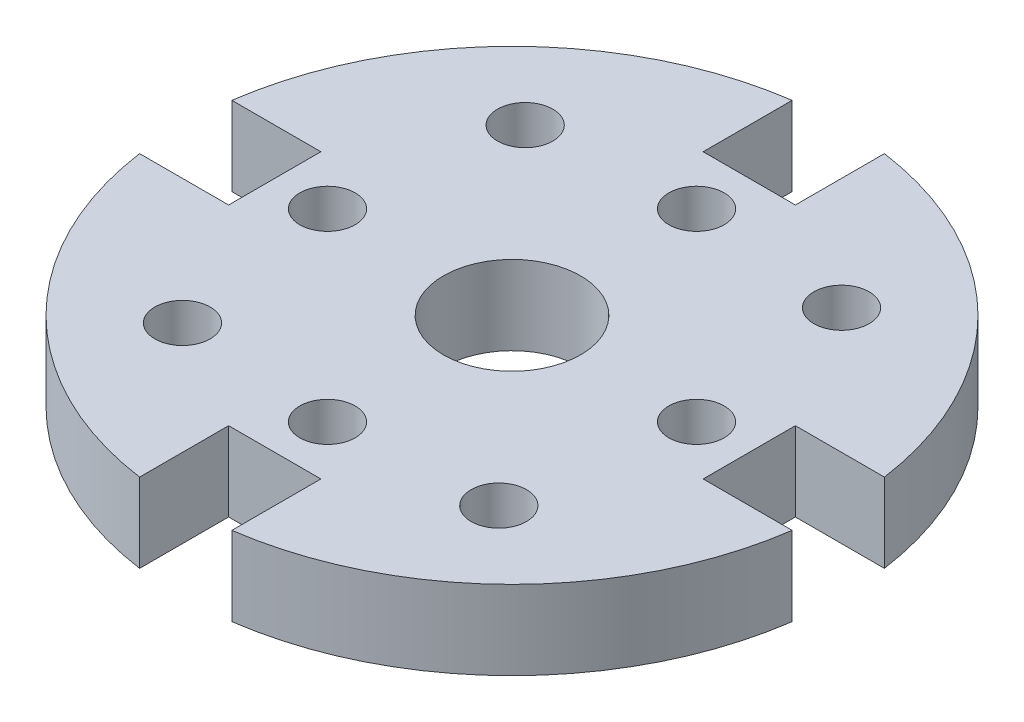
from build123d import *

# Parameters (mm, degrees)
SKETCH1_R           = 31.75
SKETCH1_R_2         = 2.667
BOSS_EXTRUDE1_DEPTH = 7.62
SKETCH2_R           = 6.604
SKETCH2_W           = 8.89
SKETCH2_H           = 17.78
CUT_EXTRUDE1_DEPTH  = 46.543269536
SKETCH3_R           = 2.667
CUT_EXTRUDE2_DEPTH  = 46.543269536
CIRPATTERN1_COUNT   = 4
SCALE1_SCALE        = 2


with BuildPart() as part:
    # Sketch1 → Boss-Extrude1 (new body)
    with BuildSketch(Plane(origin=(0, 0, 0), x_dir=(1, 0, 0), z_dir=(0, 1, 0))):
        with Locations(Location((0, 0, 0), (0, 0, 270))):
            Circle(SKETCH1_R)
        with Locations(Location((-15.24, 16.51, 0), (0, 0, 270))):
            Circle(SKETCH1_R_2, mode=Mode.SUBTRACT)
        with Locations(Location((15.24, 16.51, 0), (0, 0, 270))):
            Circle(SKETCH1_R_2, mode=Mode.SUBTRACT)
        with Locations(Location((15.24, -16.51, 0), (0, 0, 270))):
            Circle(SKETCH1_R_2, mode=Mode.SUBTRACT)
        with Locations(Location((-15.24, -16.51, 0), (0, 0, 270))):
            Circle(SKETCH1_R_2, mode=Mode.SUBTRACT)
    extrude(amount=-BOSS_EXTRUDE1_DEPTH)

    # Sketch2 → Cut-Extrude1 (cut, through all)
    with BuildSketch(Plane(origin=(0, 0, 0), x_dir=(1, 0, 0), z_dir=(0, 1, 0))):
        with Locations(Location((0, 0, 0), (0, 0, 270))):
            Circle(SKETCH2_R)
        with Locations((0, 31.75)):
            Rectangle(SKETCH2_W, SKETCH2_H)
    cut_extrude1 = extrude(amount=-CUT_EXTRUDE1_DEPTH, mode=Mode.SUBTRACT)

    # Sketch3 → Cut-Extrude2 (cut, through all)
    with BuildSketch(Plane(origin=(0, 0, 0), x_dir=(1, 0, 0), z_dir=(0, 1, 0))):
        with Locations(Location((-17.78, 0, 0), (0, 0, 270))):
            Circle(SKETCH3_R)
        with Locations(Location((0, 17.78, 0), (0, 0, 270))):
            Circle(SKETCH3_R)
        with Locations(Location((17.78, 0, 0), (0, 0, 270))):
            Circle(SKETCH3_R)
        with Locations(Location((0, -17.78, 0), (0, 0, 270))):
            Circle(SKETCH3_R)
    extrude(amount=-CUT_EXTRUDE2_DEPTH, mode=Mode.SUBTRACT)

    # CirPattern1: Cut-Extrude1 ×4 about axis
    cirpattern1_axis = Axis((0, 0, 0), (0, 1, 0))
    for i in range(1, CIRPATTERN1_COUNT):
        add(cut_extrude1.rotate(cirpattern1_axis, i * 360 / CIRPATTERN1_COUNT), mode=Mode.SUBTRACT)


with BuildPart() as part_1:
    # Scale1: scaled about (0, 0, 0)
    add(part.part.scale(SCALE1_SCALE))


solid = part_1.part
